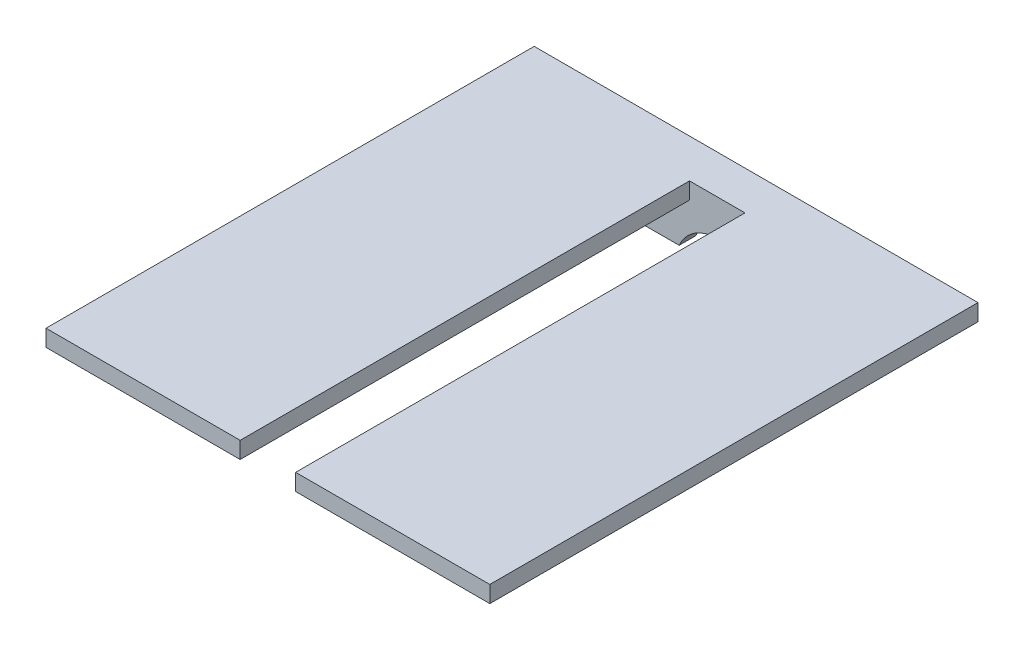
SolidWorks part; units mm, degrees
ref_plane "Front Plane" through (0, 0, 0) normal (0, 0, 1) x (1, 0, 0)
ref_plane "Top Plane" through (0, 0, 0) normal (0, 1, 0) x (1, 0, 0)
ref_plane "Right Plane" through (0, 0, 0) normal (1, 0, 0) x (0, 0, -1)
sketch "Sketch2" plane through (0, 0, 0) normal (0, 0, 1) x (1, 0, 0)
  line L0 (-20, 3) -> (-6.8739, 3)
  line L2 (-20, 3) -> (-20, 11)
  line L3 (-20, 11) -> (20, 11)
  line L4 (20, 3) -> (20, 11)
  line L7 (6.8739, 3) -> (20, 3)
  circle A0 centre (-17, 7) radius 1.5
  circle A1 centre (17, 7) radius 1.5
  arc A4 (6.8739, 3) -> (-6.8739, 3) centre (0, 0) ccw
  point P0 (0, 0)
  dimension "D1" = 3
  dimension "D2" = 3
  dimension "D3" = 40
  dimension "D4" = 8
  dimension "D9" = 3
  dimension "D11" = 15
  dimension "D5" = 20
  dimension "D8" = 3
extrude "Boss-Extrude1" add sketch "Sketch2" along normal blind 3
sketch "Sketch3" plane through (0, 11, 0) normal (0, 1, 0) x (1, 0, 0)
  line L0 (-5, -84) -> (-40, -84)
  line L2 (40, 0) -> (40, -84)
  line L3 (40, -84) -> (5, -84)
  line L4 (-40, 0) -> (-40, -84)
  line L6 (-40, 0) -> (-40, 4)
  line L7 (-40, 4) -> (40, 4)
  line L8 (40, 0) -> (40, 4)
  line L10 (-5, -3) -> (-5, -84)
  line L11 (5, -3) -> (5, -84)
  line L12 (-5, -3) -> (5, -3)
  line L13 (20, -3) -> (-20, -3) construction
  dimension "D1" = 84
  dimension "D2" = 80
  dimension "D3" = 4
  dimension "D4" = 40
  dimension "D5" = 0
extrude "Boss-Extrude2" add sketch "Sketch3" along normal blind 3
